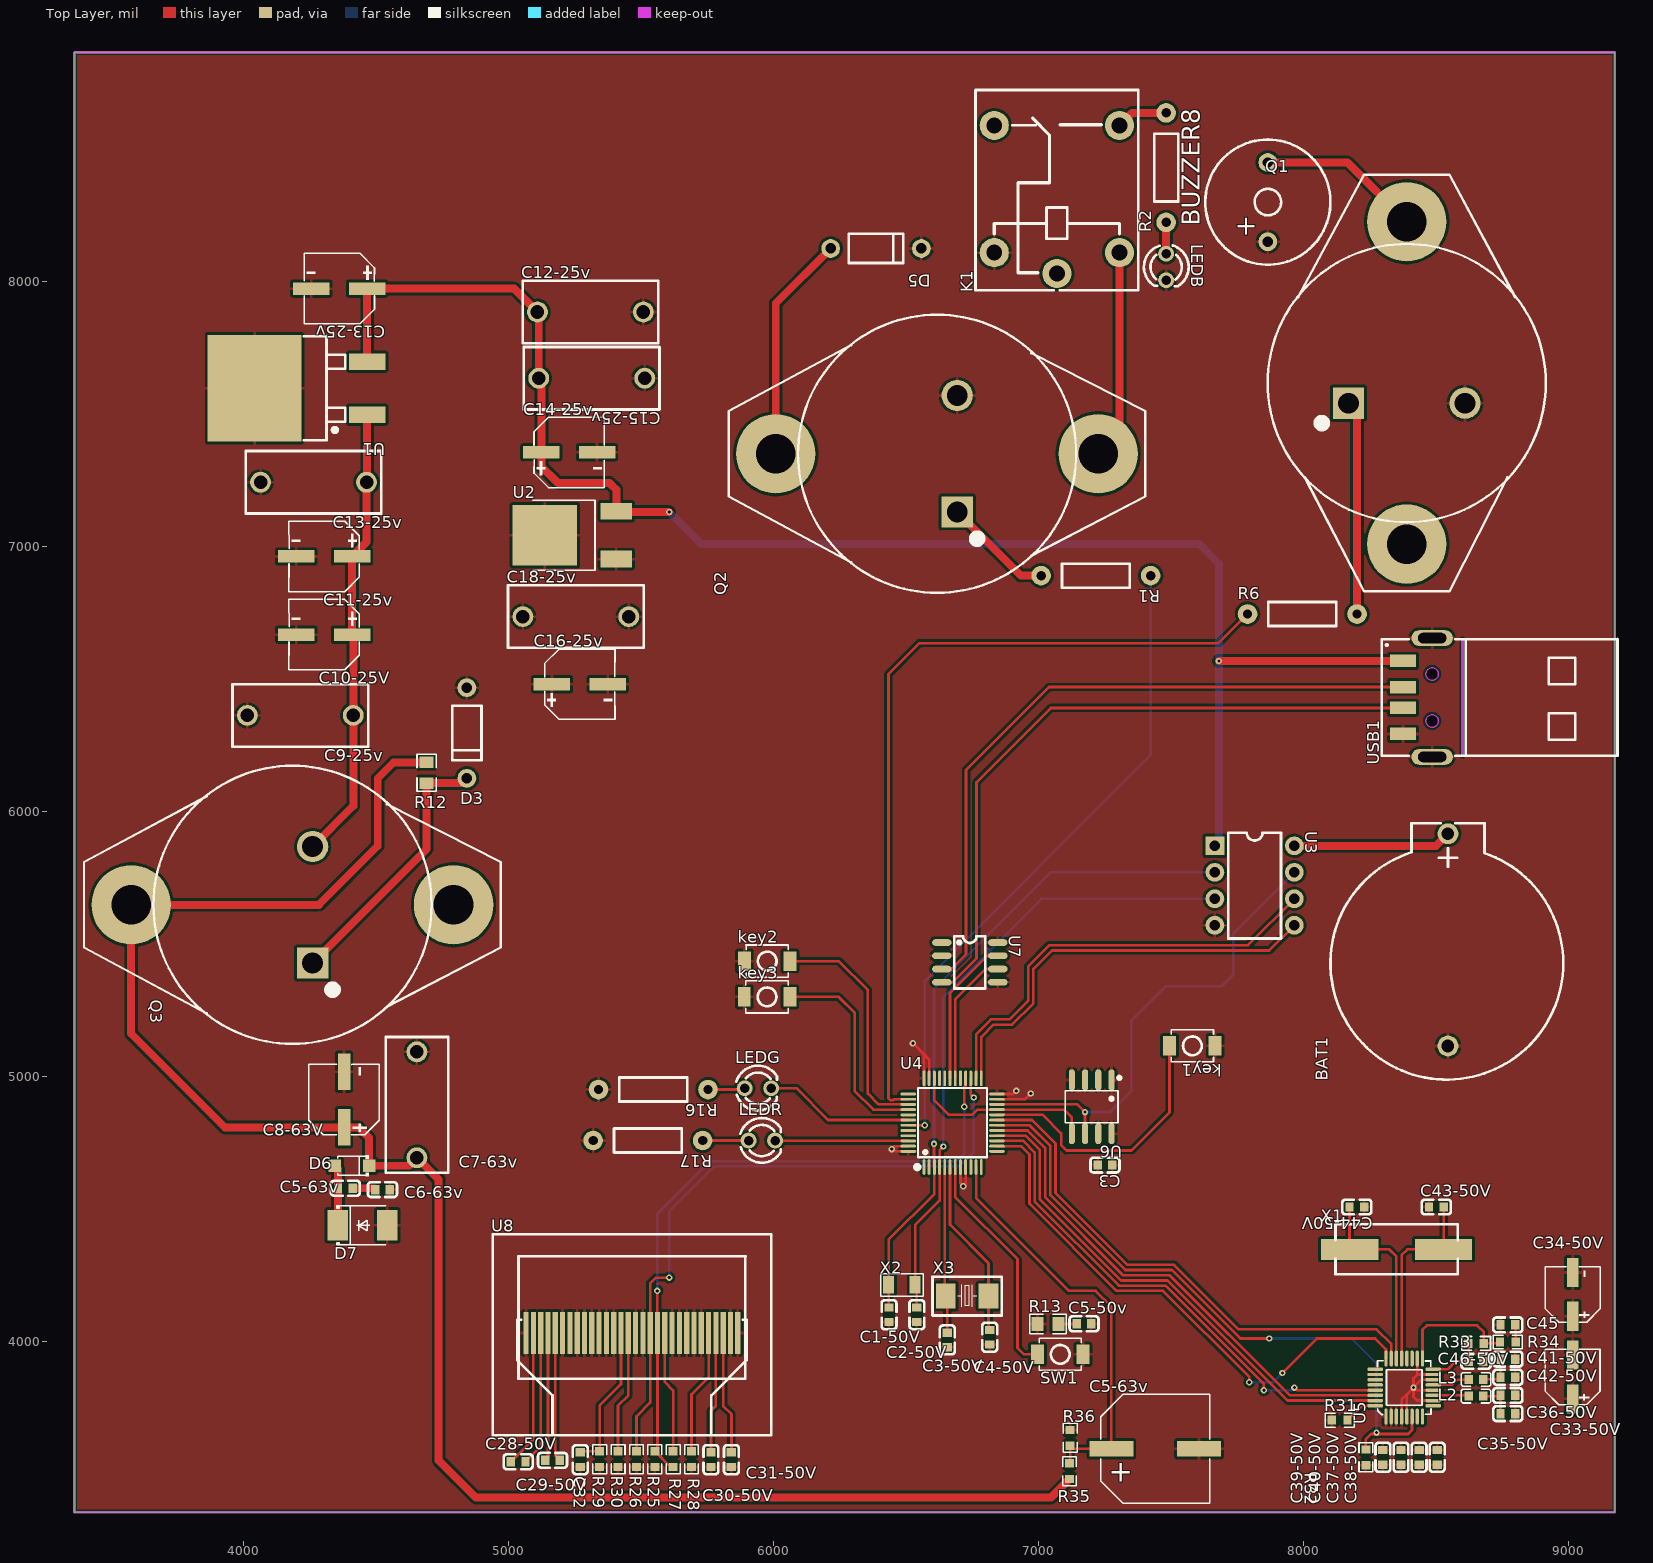
[diagram p0: Top Layer view]
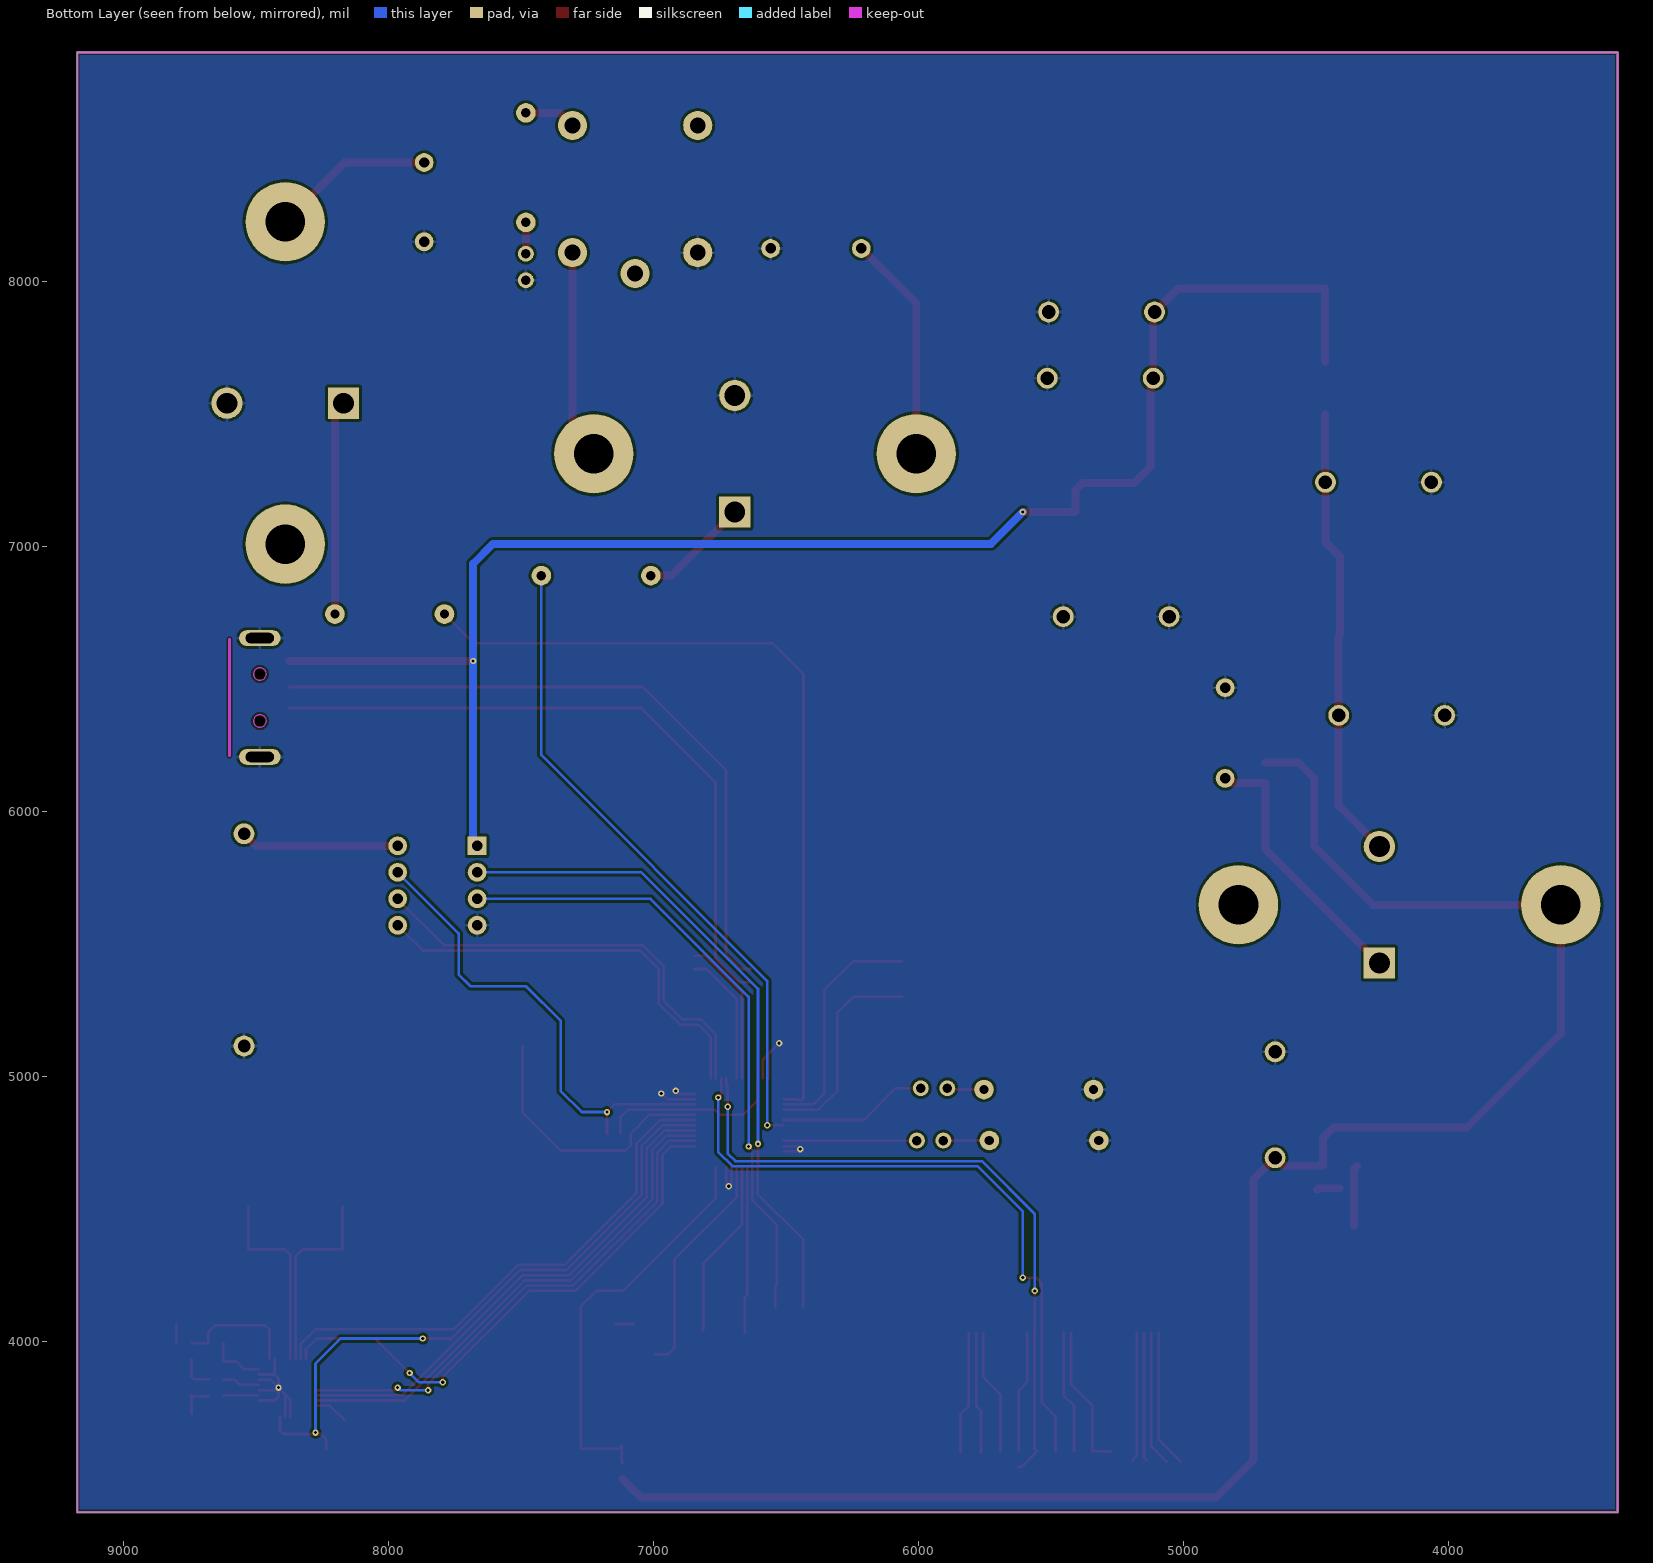
[diagram p1: Bottom Layer view, seen from below]
# Altium PCB MISC52145.pcbdoc
Units mil, origin at the board's own origin, x right, y up, seen from the top; angles counter-clockwise.
Board outline 5815 x 5510 mil, 2 copper layers (Top Layer, Bottom Layer), stack 62.206 mil thick; 90 components, 71 nets, 317 pads, 22 vias.

## Layer stack, top to bottom
Top Solder Mask Layer: solder mask 0.394, Dk 3.3
Top Layer: signal copper 1.379
Dielectric1: surface 59.449, FR4, Dk 4.5
Bottom Layer: signal copper 1.378
Bottom Solder Mask Layer: solder mask 0.394, Dk 3.3

## Board outline
3360,8865 3360,3355 9175,3355 9175,8865

## Design rules (kind name [scope] priority, off if disabled: settings)
BoardOutlineClearance copperThickness2oz_1 [All] p2 off: genericclearance=7.99 ignorepadtopadclearanceinfootprint=FALSE except(0: Arc-SplitContinuation Track-SplitContinuation SMDPad-SplitContinuation THPad-SplitContinuation Via-SplitContinuation Fill-SplitContinuation Region-SplitContinuation Poly-SplitContinuation Text-SplitContinuation Hole-SplitContinuation; 5.98: Arc-CutoutEdge SMDPad-CutoutEdge THPad-CutoutEdge Via-CutoutEdge Fill-CutoutEdge Region-CutoutEdge Text-CutoutEdge; 6.93: Hole-OutlineEdge Hole-CutoutEdge; 10: Poly-OutlineEdge Poly-CutoutEdge; 11.81: Arc-OutlineEdge Track-OutlineEdge SMDPad-OutlineEdge THPad-OutlineEdge Via-OutlineEdge Fill-OutlineEdge Region-OutlineEdge Text-OutlineEdge Track-CutoutEdge)
BoardOutlineClearance Plane_innerPlane_1 [All] p4 off: genericclearance=4.02 ignorepadtopadclearanceinfootprint=FALSE except(0: Arc-SplitContinuation Track-SplitContinuation SMDPad-SplitContinuation THPad-SplitContinuation Via-SplitContinuation Fill-SplitContinuation Region-SplitContinuation Poly-SplitContinuation Text-SplitContinuation Hole-SplitContinuation; 6: SMDPad-CutoutEdge THPad-CutoutEdge Via-CutoutEdge Fill-CutoutEdge Region-CutoutEdge Text-CutoutEdge; 6.93: Hole-OutlineEdge Hole-CutoutEdge; 10: Poly-OutlineEdge Poly-CutoutEdge; 11.8: Arc-OutlineEdge Track-OutlineEdge SMDPad-OutlineEdge THPad-OutlineEdge Via-OutlineEdge Fill-OutlineEdge Region-OutlineEdge Text-OutlineEdge; 11.81: Arc-CutoutEdge Track-CutoutEdge)
BoardOutlineClearance Copper_copperRegion_1 [All] p6 off: genericclearance=4.02 ignorepadtopadclearanceinfootprint=FALSE except(0: Arc-SplitContinuation Track-SplitContinuation SMDPad-SplitContinuation THPad-SplitContinuation Via-SplitContinuation Fill-SplitContinuation Region-SplitContinuation Poly-SplitContinuation Text-SplitContinuation Hole-SplitContinuation; 6: SMDPad-CutoutEdge THPad-CutoutEdge Via-CutoutEdge Fill-CutoutEdge Region-CutoutEdge Text-CutoutEdge; 6.93: Hole-OutlineEdge Hole-CutoutEdge; 10: Poly-OutlineEdge Poly-CutoutEdge; 11.8: Arc-OutlineEdge Track-OutlineEdge SMDPad-OutlineEdge THPad-OutlineEdge Via-OutlineEdge Fill-OutlineEdge Region-OutlineEdge Text-OutlineEdge; 11.81: Arc-CutoutEdge Track-CutoutEdge)
BoardOutlineClearance copperThickness1oz_1 [All] p8: genericclearance=4.02 ignorepadtopadclearanceinfootprint=FALSE except(0: Arc-SplitContinuation Track-SplitContinuation SMDPad-SplitContinuation THPad-SplitContinuation Via-SplitContinuation Fill-SplitContinuation Region-SplitContinuation Poly-SplitContinuation Text-SplitContinuation Hole-SplitContinuation; 6: SMDPad-CutoutEdge THPad-CutoutEdge Via-CutoutEdge Fill-CutoutEdge Region-CutoutEdge Text-CutoutEdge; 6.93: Hole-OutlineEdge Hole-CutoutEdge; 10: Poly-OutlineEdge Poly-CutoutEdge; 11.8: Arc-OutlineEdge Track-OutlineEdge SMDPad-OutlineEdge THPad-OutlineEdge Via-OutlineEdge Fill-OutlineEdge Region-OutlineEdge Text-OutlineEdge; 11.81: Arc-CutoutEdge Track-CutoutEdge)
Clearance copperThickness2oz [All] p1 off: gap=7.99 ignorepadtopadclearanceinfootprint=FALSE except(5.98: SMDPad-Track SMDPad-SMDPad THPad-Track SMDPad-THPad THPad-THPad Track-Via SMDPad-Via THPad-Via Via-Via Fill-Track Region-Track Fill-SMDPad Region-SMDPad Fill-THPad Region-THPad Fill-Via Region-Via Fill-Fill Fill-Region Region-Region Arc-Track Arc-SMDPad Arc-THPad Arc-Via Fill-Arc Region-Arc Arc-Arc Text-Track SMDPad-Text Text-THPad Text-Via Fill-Text Region-Text Arc-Text Text-Text; 6.93: Hole-Track Hole-SMDPad Hole-THPad Hole-Via Fill-Hole Region-Hole Hole-Arc Hole-Text; 10: Poly-Track Poly-SMDPad Poly-THPad Poly-Via Poly-Fill Poly-Region Poly-Poly Poly-Arc Poly-Text Poly-Hole)
Clearance Plane_innerPlane [All] p3 off: gap=4.02 ignorepadtopadclearanceinfootprint=FALSE except(5.98: SMDPad-Track SMDPad-SMDPad THPad-Track SMDPad-THPad THPad-THPad Track-Via SMDPad-Via THPad-Via Via-Via Fill-Track Region-Track Fill-SMDPad Region-SMDPad Fill-THPad Region-THPad Fill-Via Region-Via Fill-Fill Fill-Region Region-Region; 6: Arc-Track Arc-SMDPad Arc-THPad Arc-Via Fill-Arc Region-Arc Arc-Arc Text-Track SMDPad-Text Text-THPad Text-Via Fill-Text Region-Text Arc-Text Text-Text; 6.93: Hole-Track Hole-SMDPad Hole-THPad Hole-Via Fill-Hole Region-Hole Hole-Arc Hole-Text; 10: Poly-Track Poly-SMDPad Poly-THPad Poly-Via Poly-Fill Poly-Region Poly-Poly Poly-Arc Poly-Text Poly-Hole)
Clearance Copper_copperRegion [All] p5 off: gap=4.02 ignorepadtopadclearanceinfootprint=FALSE except(5.98: SMDPad-Track SMDPad-SMDPad THPad-Track SMDPad-THPad THPad-THPad Track-Via SMDPad-Via THPad-Via Via-Via Fill-Track Region-Track Fill-SMDPad Region-SMDPad Fill-THPad Region-THPad Fill-Via Region-Via Fill-Fill Fill-Region Region-Region; 6: Arc-Track Arc-SMDPad Arc-THPad Arc-Via Fill-Arc Region-Arc Arc-Arc Text-Track SMDPad-Text Text-THPad Text-Via Fill-Text Region-Text Arc-Text Text-Text; 6.93: Hole-Track Hole-SMDPad Hole-THPad Hole-Via Fill-Hole Region-Hole Hole-Arc Hole-Text; 10: Poly-Track Poly-SMDPad Poly-THPad Poly-Via Poly-Fill Poly-Region Poly-Poly Poly-Arc Poly-Text Poly-Hole)
Clearance copperThickness1oz [All] p7: gap=4.02 ignorepadtopadclearanceinfootprint=FALSE except(5.98: SMDPad-Track SMDPad-SMDPad THPad-Track SMDPad-THPad THPad-THPad Track-Via SMDPad-Via THPad-Via Via-Via Fill-Track Region-Track Fill-SMDPad Region-SMDPad Fill-THPad Region-THPad Fill-Via Region-Via Fill-Fill Fill-Region Region-Region; 6: Arc-Track Arc-SMDPad Arc-THPad Arc-Via Fill-Arc Region-Arc Arc-Arc Text-Track SMDPad-Text Text-THPad Text-Via Fill-Text Region-Text Arc-Text Text-Text; 6.93: Hole-Track Hole-SMDPad Hole-THPad Hole-Via Fill-Hole Region-Hole Hole-Arc Hole-Text; 10: Poly-Track Poly-SMDPad Poly-THPad Poly-Via Poly-Fill Poly-Region Poly-Poly Poly-Arc Poly-Text Poly-Hole)
DiffPairsRouting differentialPair [All] p1: maxlimit=6 minlimit=6 mostfreqgap=6 toplayer_minwidth=5 toplayer_prefwidth=10 toplayer_maxwidth=100 toplayer_mingap=6 toplayer_prefgap=6 toplayer_maxgap=6 bottomlayer_minwidth=5 bottomlayer_prefwidth=10 bottomlayer_maxwidth=100 bottomlayer_mingap=6 bottomlayer_prefgap=6 bottomlayer_maxgap=6 maxuncoupledlength=10
HoleToHoleClearance otherClearance [All] p1: gap=11.81 allowstackedmicrovias=TRUE
Length netLength [All] p1: minlimit=0 maxlimit=0
PasteMaskExpansion pasteMaskExpansion [All] p1: expansion=0
PlaneConnect innerPlane [All] p1: planeconnectstyle=Relief reliefexpansion=20 reliefentries=4 reliefconductorwidth=10 reliefairgap=10
PolygonConnect copperRegion [(InNet('GND'))] p1: connectstyle=Relief reliefconductorwidth=10 reliefentries=4 polygonreliefangle="90 Angle" airgapwidth=10 via.connectstyle=Relief via.reliefconductorwidth=10 via.reliefentries=4 via.polygonreliefangle="90 Angle" via.airgapwidth=10
RoutingVias viaSize [All] p1: holewidth=12.01 width=24.02 viastyle="Through Hole" minholewidth=11.81 minwidth=19.68 maxholewidth=248.03 maxwidth=393.7
SolderMaskExpansion solderMaskExpansion [IsVia] p1: expansion=-1000 istentingtop=TRUE
SolderMaskExpansion solderMaskExpansion [All] p2: expansion=2 istentingtop=FALSE
Width copperThickness2oz_2 [All] p1 off: maxlimit=100 minlimit=8 preferedwidth=10
Width copperThickness1oz_2 [All] p2: maxlimit=100 minlimit=5 preferedwidth=10

## Components (designator, comment, footprint, x,y, rotation, side; value= is the part's Value field where it differs from the comment)
BAT1 "CR2032-2-1" BAT-TH_CR2032-2-1 8545,5515 r90 top
BUZZER8 "buzzer-12X9" BUZ-TH_BD12.0-P7.60-D0.6-FD 7865,8300 r90 top
C1-50V "22pF" C0603 6435,4100 r270 top
C2-50V "22pF" C0603 6540,4100 r270 top
C3 "100nF" C0603 7250,4665 r180 top
C3-50V "22pF" C0603 6655,4005 r270 top
C4-50V "22pF" C0603 6815,4015 r270 top
C5-50v "100nF" C0603 7171.16,4065.82 r0 top
C5-63v "100uF" CAP-SMD_BD10.0-L10.3-W10.3-LS11.0-FD_1 7439.75,3593.72 r0 top
C5-63v "100nF" C0603 4382.66,4577.44 r180 top
C6-63v "100nF" C0603 4522.66,4572.44 r180 top
C7-63v "100nF" CAP-TH_L13.0-W6.0-P10.00-D1.0 4652.66,4892.44 r90 top
C8-63V "100uF" CAP-SMD_BD6.3-L6.6-W6.6-LS7.3-FD-H7.7 4377.66,4912.44 r90 top
C9-25v "100nF" CAP-TH_L13.0-W6.0-P10.00-D1.0 4212.66,6362.44 r180 top
C10-25V "100uF" CAP-SMD_BD6.3-L6.6-W6.6-LS7.3-FD-H7.7 4302.66,6667.44 r180 top
C11-25v "100uF" CAP-SMD_BD6.3-L6.6-W6.6-LS7.3-FD-H7.7 4302.66,6962.44 r180 top
C12-25v "100nF" CAP-TH_L13.0-W6.0-P10.00-D1.0 5307.66,7885.24 r0 top
C13-25v "100uF" CAP-SMD_BD6.3-L6.6-W6.6-LS7.3-FD-H7.7 4359.68,7973.62 r180 top
C13-25v "100nF" CAP-TH_L13.0-W6.0-P10.00-D1.0 4262.66,7242.44 r180 top
C14-25v "100uF" CAP-SMD_BD6.3-L6.6-W6.6-LS7.3-FD-H7.7 5227.66,7355.24 r0 top
C15-25v "100nF" CAP-TH_L13.0-W6.0-P10.00-D1.0 5312.66,7635.24 r180 top
C16-25v "100uF" CAP-SMD_BD6.3-L6.6-W6.6-LS7.3-FD-H7.7 5267.66,6480.24 r0 top
C18-25v "100nF" CAP-TH_L13.0-W6.0-P10.00-D1.0 5252.66,6735.24 r0 top
C28-50V "1uF" C0603 5035,3545 r180 top
C29-50V "1uF" C0603 5164.81,3550.37 r180 top
C30-50V "4.7uF" C0603 5762.84,3552.81 r90 top
C31-50V "2.2uF" C0603 5840.08,3552.81 r90 top
C32 "10uF" C0603 5269.49,3552.81 r90 top
C33-50V "0.1uF" CAP-SMD_BD5.0-L5.3-W5.3-FD 9015.85,3865.07 r90 top
C34-50V "0.1uF" CAP-SMD_BD5.0-L5.3-W5.3-FD 9015.91,4176.73 r90 top
C35-50V "47pF" C0603 8770.92,3795.31 r180 top
C36-50V "15pF" C0603 8770.91,3726.73 r0 top
C37-50V "180pF" C0603 8435.96,3561.73 r90 top
C38-50V "10pF" C0603 8504.27,3561.73 r90 top
C39-50V "180pF" C0603 8299.36,3561.73 r90 top
C40-50V "10pF" C0603 8367.66,3561.73 r90 top
C41-50V "15pF" C0603 8770.91,3932.47 r0 top
C42-50V "47pF" C0603 8770.91,3863.89 r0 top
C43-50V "15pF" C0603 8500.91,4506.73 r0 top
C44-50V "15pF" C0603 8200.91,4506.73 r180 top
C45 "0.1uF" C0603 8770.91,4061.73 r0 top
C46-50V "0.1uF" C0603 8650.91,3923.61 r0 top
D3 "1N4742A" DO-41_BD2.4-L4.7-P8.70-D0.9-RD 4841.4,6295.87 r90 top
D5 "1N4003-E3/54" DO-41_BD2.4-L4.7-P8.70-D0.9-RD 6385.95,8125.05 r180 top
D6 "1N4003W" SOD-123FL_L2.7-W1.8-LS3.8-RD 4407.66,4662.44 r180 top
D7 "SMBJ51A" SMB_L4.3-W3.6-LS5.4-R-RD 4447.66,4437.44 r0 top
K1 "" RELAY-TH_SRD-DCXXV-SL-C 7068.54,8310.03 r90 top
key1 "TS-1088-AR02016" SW-SMD_L3.9-W3.0-P4.45 7580,5115 r180 top
key2 "TS-1088-AR02016" SW-SMD_L3.9-W3.0-P4.45 5975,5435 r0 top
key3 "TS-1088-AR02016" SW-SMD_L3.9-W3.0-P4.45 5974.59,5299.8 r0 top
L2 "2.2uH" L0603 8650.91,3792.51 r0 top
L3 "2.2uH" L0603 8650.91,3855.91 r0 top
LEDB "" LED_TH-3mm 7480.95,8055.05 r270 top
LEDG "" LED_TH-3mm 5940,4955 r0 top
LEDR "" LED_TH-3mm 5954.79,4757.59 r0 top
Q1 "2N3055" TO-3_L39.4-W26.7-P10.92-BL 8389.2,7617.41 r0 top
Q2 "2N3055" TO-3_L39.4-W26.7-P10.92-BL 6615.95,7350.05 r90 top
Q3 "2N3055" TO-3_L39.4-W26.7-P10.92-BL 4182.66,5647.44 r90 top
R1 "" RES-TH_BD2.3-L6.5-P10.50-D0.5 7215.95,6890.05 r180 top
R2 "" RES-TH_BD2.3-L6.5-P10.50-D0.5 7480.95,8430.05 r90 top
R6 "" RES-TH_BD2.3-L6.5-P10.50-D0.5 7995,6745 r0 top
R12 "10kΩ" R0805 4689.17,6145.87 r90 top
R13 "10kΩ" R0805 7035,4065 r0 top
R16 "" RES-TH_BD2.3-L6.5-P10.50-D0.5 5545,4950 r180 top
R17 "" RES-TH_BD2.3-L6.5-P10.50-D0.5 5524.79,4757.63 r180 top
R25 "4.7K" R0603 5550.84,3555 r270 top
R26 "4.7K" R0603 5481.49,3555 r270 top
R27 "0" R0603 5620.19,3555 r90 top
R28 "910K" R0603 5689.54,3555 r90 top
R29 "10K" R0603 5342.79,3555 r270 top
R30 "10K" R0603 5412.14,3555 r270 top
R31 "1K" R0603 8135.91,3701.73 r0 top
R32 "10k" R0603 8235,3561.73 r270 top
R33 "820Ω" R0603 8650.91,3991.73 r0 top
R34 "5.1k" R0603 8770.92,3997.1 r0 top
R35 "30kΩ" R0603 7116.37,3509.66 r90 top
R36 "1kΩ" R0603 7118.81,3635.34 r270 top
SW1 "TS-1088-AR02016" SW-SMD_L3.9-W3.0-P4.45 7081.16,3950.56 r0 top
U1 "L7805ABD2T-TR" TO-263-2_L10.0-W9.2-P5.08-LS15.3-TL-CW 4252.66,7597.44 r180 top
U2 "LD1117DT33TR" TO-252-2_L6.6-W6.1-P4.57-LS9.9-BR-CW 5270.71,7042.64 r0 top
U3 "DS1302" DIP-8_L9.7-W6.4-P2.54-LS7.6-BL 7815,5720 r270 top
U4 "STM32F103C8T6" LQFP-48_L7.0-W7.0-P0.50-LS9.0-BL 6675,4825 r0 top
U5 "MFRC522" QFN32 8310.91,3716.73 r90 top
U6 "AT24C02" SOIC-8_L4.9-W3.9-P1.27-LS6.0-BL 7200,4885 r180 top
U7 "CH340N" SOP-8_L4.9-W3.9-P1.27-LS6.0-BL 6740,5430 r270 top
U8 "X096-2864KLBAG01-H30" OLED-SMD_X096-2864KLBAG01-H30 5464.46,4030.95 r0 top
USB1 "U217-041N-4BV81" USB-A-SMD_U217-041N-4BV81 8430,6430 r90 top
X1 "27.12MHz" OSC-SMD_L11.4-W4.5-LS12.5 8350.91,4346.73 r0 top
X2 "32.768kHz" CRYSTAL-SMD_L3.2-W1.5-1 6483.58,4212.95 r180 top
X3 "8MHz" CRYSTAL-SMD_L5.0-W3.2 6730,4170 r180 top

## Footprints (in the part's own frame and the unit in brackets; to place one, negate y for a bottom-side part, rotate by r counter-clockwise, add the part's x,y. Pads: shape width x height; smd on the part's side, far side on the other; paste and mask are expansions set on the pad)
BAT-TH_CR2032-2-1 [mm]
  round 2 hole 1.2 paste+0 mask+0.051: 1(10.175,0) 2(-10.175,0)
  silkscreen extent -13.4,-11.05 11.17,11.26
BUZ-TH_BD12.0-P7.60-D0.6-FD [mil]
  round 70.9 hole 39.4 paste+0 mask+2: 1(-149.6,0) 2(149.6,0)
  silkscreen extent -236,-236 236,236
C0603 [mm]
  rect 0.8x0.9 smd: 1(-0.7,0) 2(0.7,0)
  silkscreen extent -1.39,-0.71 1.39,0.71
CAP-SMD_BD5.0-L5.3-W5.3-FD [mm]
  rect 2.8x1.1 smd: 1(-2.1,0) 2(2.1,0)
  silkscreen extent -2.66,-2.62 2.66,2.65
CAP-SMD_BD6.3-L6.6-W6.6-LS7.3-FD-H7.7 [mm]
  rect 3.5x1.2 smd: 1(-2.67,0) 2(2.67,0)
  silkscreen extent -3.38,-3.38 3.38,3.38
CAP-SMD_BD10.0-L10.3-W10.3-LS11.0-FD_1 [mm]
  rect 4.2x1.5 smd: 1(-4.2,0) 2(4.2,0)
  silkscreen extent -5.23,-5.23 5.23,5.23
CAP-TH_L13.0-W6.0-P10.00-D1.0 [mm]
  round 2 hole 1.3: 1(-5.08,0) 2(5.08,0)
  silkscreen extent -6.5,-3 6.5,3
CRYSTAL-SMD_L3.2-W1.5-1 [mm]
  rect 1.05x1.7 smd: 1(-1.275,0) 2(1.275,0)
  silkscreen extent -2.03,-1.08 2.03,1.08
CRYSTAL-SMD_L5.0-W3.2 [mm]
  rect 1.9x2.4 smd: 1(-2.05,0) 2(2.05,0)
  silkscreen extent -3.32,-1.85 3.33,1.85
DIP-8_L9.7-W6.4-P2.54-LS7.6-BL [mm]
  rect 1.8x1.8 hole 1 paste+0 mask+0.05: 1(-3.81,-3.81)
  round 1.8 hole 1 paste+0 mask+0.05: 2(-1.27,-3.81) 3(1.27,-3.81) 4(3.81,-3.81) 5(3.81,3.81) 6(1.27,3.81) 7(-1.27,3.81) 8(-3.81,3.81)
  silkscreen extent -5.08,-2.53 5.08,2.53
DO-41_BD2.4-L4.7-P8.70-D0.9-RD [mm]
  round 1.8 hole 1: 1(-4.35,0) 2(4.35,0)
  silkscreen extent -2.6,-1.4 2.6,1.4
L0603 [mm]
  rect 0.8x0.864 smd paste-100 mask+0.051: 1(-0.7,0) 2(0.7,0)
  silkscreen extent -1.42,-0.65 1.42,0.65
LED_TH-3mm [mil]
  round 60 hole 36 paste+0 mask+2: 1(-50,0) 2(50,0)
  silkscreen extent -81,-84 72,85
LQFP-48_L7.0-W7.0-P0.50-LS9.0-BL [mm]
  oval 0.27x1.5 smd paste+0 mask+0.05: 1(-2.75,-4.25) 2(-2.25,-4.25) 3(-1.75,-4.25) 4(-1.25,-4.25) 5(-0.75,-4.25) 6(-0.25,-4.25) 7(0.25,-4.25) 8(0.75,-4.25) 9(1.25,-4.25) 10(1.75,-4.25) 11(2.25,-4.25) 12(2.75,-4.25) 25(2.75,4.25) 26(2.25,4.25) 27(1.75,4.25) 28(1.25,4.25) 29(0.75,4.25) 30(0.25,4.25) 31(-0.25,4.25) 32(-0.75,4.25) 33(-1.25,4.25) 34(-1.75,4.25) 35(-2.25,4.25) 36(-2.75,4.25)
  oval 1.5x0.27 smd paste+0 mask+0.05: 13(4.25,-2.75) 14(4.25,-2.25) 15(4.25,-1.75) 16(4.25,-1.25) 17(4.25,-0.75) 18(4.25,-0.25) 19(4.25,0.25) 20(4.25,0.75) 21(4.25,1.25) 22(4.25,1.75) 23(4.25,2.25) 24(4.25,2.75) 37(-4.25,2.75) 38(-4.25,2.25) 39(-4.25,1.75) 40(-4.25,1.25) 41(-4.25,0.75) 42(-4.25,0.25) 43(-4.25,-0.25) 44(-4.25,-0.75) 45(-4.25,-1.25) 46(-4.25,-1.75) 47(-4.25,-2.25) 48(-4.25,-2.75)
  silkscreen extent -3.59,-4.46 3.3,3.34
OLED-SMD_X096-2864KLBAG01-H30 [mm]
  rect 0.5x4 smd: 1(-10.15,0) 2(-9.45,0) 3(-8.75,0) 4(-8.05,0) 5(-7.35,0) 6(-6.65,0) 7(-5.95,0) 8(-5.25,0) 9(-4.55,0) 10(-3.85,0) 11(-3.15,0) 12(-2.45,0) 13(-1.75,0) 14(-1.05,0) 15(-0.35,0) 16(0.35,0) 17(1.05,0) 18(1.75,0) 19(2.45,0) 20(3.15,0) 21(3.85,0) 22(4.55,0) 23(5.25,0) 24(5.95,0) 25(6.65,0) 26(7.35,0) 27(8.05,0) 28(8.75,0) 29(9.45,0) 30(10.15,0)
  silkscreen extent -13.35,-9.8 13.35,9.46
OSC-SMD_L11.4-W4.5-LS12.5 [mm]
  rect 5.5x2 smd: 1(-4.5,0) 2(4.5,0)
  silkscreen extent -5.85,-2.4 5.85,2.4
QFN32 [mil]
  oval 60x13 smd: 1(-1,0) 2(-1,-20) 3(-1,-39.39) 4(-1,-59.08) 5(-1,-78.76) 6(-1,-98.45) 7(-1,-118.15) 8(-1,-137.84) 17(218,-137.84) 18(218,-118.15) 19(218,-98.45) 20(218,-78.76) 21(218,-59.08) 22(218,-39.39) 23(218,-20) 24(218,0)
  oval 13x60 smd: 9(39.59,-178.42) 10(59.28,-178.42) 11(78.97,-178.42) 12(98.66,-178.42) 13(118.35,-178.42) 14(138.04,-178.42) 15(157.73,-178.42) 16(177.38,-178.42) 25(177.38,40.58) 26(157.73,40.58) 27(138.04,40.58) 28(118.35,40.58) 29(98.66,40.58) 30(78.97,40.58) 31(59.28,40.58) 32(39.59,40.58)
  silkscreen extent 6,-169 210,32
R0603 [mil]
  rect 31.75x34.02 smd paste-3937.01 mask+2: 1(-29.66,0) 2(29.66,0)
  silkscreen extent -55,-26 55,26
R0805 [mm]
  rect 1.133x1.377 smd paste-100 mask+0.051: 1(-1,0) 2(1,0)
  silkscreen extent -1.76,-0.92 1.76,0.92
RELAY-TH_SRD-DCXXV-SL-C [mil]
  round 110 hole 60 paste+0 mask+2: 1(-200.8,-236.2) 2(279.5,-236.2) 3(279.5,236.2) 4(-200.8,236.2) 5(-279.5,0)
  silkscreen extent -343,-307 413,307
RES-TH_BD2.3-L6.5-P10.50-D0.5 [mil]
  round 74 hole 35.4 paste+0 mask+2: 1(-206.69,0) 2(206.69,0)
  silkscreen extent -128,-45 128,45
SMB_L4.3-W3.6-LS5.4-R-RD [mm]
  rect 1.96x2.94 smd: 1(2.38,0) 2(-2.38,0)
  silkscreen extent -2.49,-1.88 2.23,1.88
SOD-123FL_L2.7-W1.8-LS3.8-RD [mm]
  rect 1.2x1.2 smd: 1(-1.635,0) 2(1.635,0)
  silkscreen extent -1.6,-1 1.38,1
SOIC-8_L4.9-W3.9-P1.27-LS6.0-BL [mm]
  oval 0.588x2.045 smd: 1(-1.905,-2.57) 2(-0.635,-2.57) 3(0.635,-2.57) 4(1.905,-2.57) 5(1.905,2.57) 6(0.635,2.57) 7(-0.635,2.57) 8(-1.905,2.57)
  silkscreen extent -2.8,-2.92 2.53,1.52
SOP-8_L4.9-W3.9-P1.27-LS6.0-BL [mm]
  oval 0.63x1.865 smd: 1(-1.905,-2.682) 2(-0.635,-2.682) 3(0.635,-2.682) 4(1.905,-2.682) 5(1.905,2.682) 6(0.635,2.682) 7(-0.635,2.682) 8(-1.905,2.682)
  silkscreen extent -2.5,-1.5 2.5,1.48
SW-SMD_L3.9-W3.0-P4.45 [mm]
  rect 1.23x1.86 smd: 1(-2.185,0) 2(2.185,0)
  silkscreen extent -2.03,-1.54 2.03,1.54
TO-3_L39.4-W26.7-P10.92-BL [mil]
  rect 118.11x118.11 hole 78.74: 1(-220,-76.5)
  round 118.11 hole 78.74: 2(220,-76.5)
  round 300 hole 150: 3(0,608.5) 4(0,-608.5)
  silkscreen extent -525,-786 525,786
TO-252-2_L6.6-W6.1-P4.57-LS9.9-BR-CW [mm]
  rect 3x1.6 smd: 1(3.424,-2.29) 3(3.424,2.29)
  rect 6.2x5.8 smd: 2(-3.424,0)
  silkscreen extent -4.58,-3.35 1.38,3.35
TO-263-2_L10.0-W9.2-P5.08-LS15.3-TL-CW [mm]
  rect 3.5x1.6 smd: 1(-5.397,2.54) 3(-5.397,-2.54)
  rect 9x10.2 smd: 2(5.397,0)
  silkscreen extent -3.3,-5 0.67,5
USB-A-SMD_U217-041N-4BV81 [mil]
  rect 47.2x98.4 smd paste-3937.01 mask+2: 1(137.8,55.1) 2(39.4,55.1) 3(-39.4,55.1) 4(-137.8,55.1)
  oval 59.1x157.5 hole 39.4 slot 106.3 at 90 deg paste+0 mask+2: 5(-224.4,-55.1) 6(224.4,-55.1)
  Board Outline Layer circle w0.1: c-88.6,-55.1 r23.6
  Board Outline Layer circle w0.1: c88.6,-55.1 r23.6
  Board Outline Layer lines w10: -220,-170 220,-170
  Board Outline Layer region: -88.6,-78.7 -98.84,-76.36 -107.05,-69.81 -111.61,-60.35 -111.61,-49.85 -107.05,-40.39 -98.84,-33.84 -88.6,-31.5 -88.6,-31.5 -78.36,-33.84 -70.15,-40.39 -65.59,-49.85 -65.59,-60.35 -70.15,-69.81 -78.36,-76.36 -88.6,-78.7
  Board Outline Layer region: -88.6,-78.7 -92.7,-78.34 -96.67,-77.28 -100.4,-75.54 -103.77,-73.18 -106.68,-70.27 -109.04,-66.9 -110.78,-63.17 -111.84,-59.2 -112.2,-55.1 -111.84,-51 -110.78,-47.03 -109.04,-43.3 -106.68,-39.93 -103.77,-37.02 -100.4,-34.66 -96.67,-32.92 -92.7,-31.86 -88.6,-31.5 -84.5,-31.86 -80.53,-32.92 -76.8,-34.66 -73.43,-37.02 -70.52,-39.93 -68.16,-43.3 -66.42,-47.03 -65.36,-51 -65,-55.1 -65.36,-59.2 -66.42,-63.17 -68.16,-66.9 -70.52,-70.27 -73.43,-73.18 -76.8,-75.54 -80.53,-77.28 -84.5,-78.34
  Board Outline Layer region: 88.6,-78.7 78.36,-76.36 70.15,-69.81 65.59,-60.35 65.59,-49.85 70.15,-40.39 78.36,-33.84 88.6,-31.5 88.6,-31.5 98.84,-33.84 107.05,-40.39 111.61,-49.85 111.61,-60.35 107.05,-69.81 98.84,-76.36 88.6,-78.7
  Board Outline Layer region: 88.6,-78.7 84.5,-78.34 80.53,-77.28 76.8,-75.54 73.43,-73.18 70.52,-70.27 68.16,-66.9 66.42,-63.17 65.36,-59.2 65,-55.1 65.36,-51 66.42,-47.03 68.16,-43.3 70.52,-39.93 73.43,-37.02 76.8,-34.66 80.53,-32.92 84.5,-31.86 88.6,-31.5 92.7,-31.86 96.67,-32.92 100.4,-34.66 103.77,-37.02 106.68,-39.93 109.04,-43.3 110.78,-47.03 111.84,-51 112.2,-55.1 111.84,-59.2 110.78,-63.17 109.04,-66.9 106.68,-70.27 103.77,-73.18 100.4,-75.54 96.67,-77.28 92.7,-78.34
  Multi-Layer board cut-out: -88.6,-78.7 -98.84,-76.36 -107.05,-69.81 -111.61,-60.35 -111.61,-49.85 -107.05,-40.39 -98.84,-33.84 -88.6,-31.5 -88.6,-31.5 -78.36,-33.84 -70.15,-40.39 -65.59,-49.85 -65.59,-60.35 -70.15,-69.81 -78.36,-76.36 -88.6,-78.7
  Multi-Layer board cut-out: 88.6,-78.7 78.36,-76.36 70.15,-69.81 65.59,-60.35 65.59,-49.85 70.15,-40.39 78.36,-33.84 88.6,-31.5 88.6,-31.5 98.84,-33.84 107.05,-40.39 111.61,-49.85 111.61,-60.35 107.05,-69.81 98.84,-76.36 88.6,-78.7
  silkscreen extent -220,-755 221,135

## Via types
v1: diameter 24.02, hole 12, Top Layer to Bottom Layer, 22 vias

## Nets (pads, with @x,y where several pads share a name; then routed paths per layer and width w, separated by ;. In a path a pad name is that pad's centre, name@x,y a point inside that pad or via, vN(x,y) a via of type N, cw(c..) or ccw(c..) an arc to the next point about the centre after c; other vN are vias at no path point)
48V: C7-63v.1 C8-63V.1 D6.1 Q3.3 R12.2 R35.1 | length 6977.9
  Top Layer w30: R12.2 4565.24,6185.24 4505,6125 4505,5870 4282.44,5647.44 Q3.3 3574.16,5160.84 3927.68,4807.32 C8-63V.1 4432.68,4807.32 4472.03,4767.97 D6.1 4622.66,4662.44 C7-63v.1 4735,4610.1 4735,3550 4875,3410 7046.37,3410 R35.1
$1N38859: C9-25v.1 C10-25V.1 C11-25v.1 C13-25v.1@4462.66,7242.44 Q3.2 U1.1 | length 1719.4
  Top Layer w30: Q3.2 4412.66,6020.94 C9-25v.1 4412.66,6662.56 C10-25V.1 C11-25v.1 4462.66,7017.32 4462.66,7242.44 4465.16,7244.94 U1.1
$1N38873: LEDR.1 R17.1 | length 173.3
  Top Layer w10: R17.1 LEDR.1
$1N38876: Q1.1 R6.2 | length 809.4
  Top Layer w30: Q1.1 8201.69,7508.42 R6.2
$1N38881: U7.4 USB1.3 | length 2559
  Top Layer w10: U7.4 6675,5355 6765,5445 6765,6110 7045.6,6390.6 USB1.3
$1N38882: U7.3 USB1.2 | length 2588.5
  Top Layer w10: U7.3 6670,5405 6725.6,5460.6 6725.6,6155.6 7039.4,6469.4 USB1.2
$1N38894: C5-50v.1 R13.2 | length 69.6
  Top Layer w10: R13.2 7142.78,4065 C5-50v.1
$1N38907: C35-50V.2 C36-50V.1 L2.2 | length 134.6
  Top Layer w10: L2.2 8740.56,3792.51 C35-50V.2 C36-50V.1
$1N38908: L2.1 U5.11 | length 135.3
  Top Layer w10: U5.11 8620.18,3795.69 L2.1
$1N38909: C41-50V.1 C42-50V.1 L3.2 | length 136.8
  Top Layer w10: L3.2 8735.37,3855.91 C42-50V.1 C41-50V.1
$1N38910: L3.1 U5.13 | length 142.7
  Top Layer w10: U5.13 8560.07,3835.07 8580,3855 8622.45,3855 L3.1
$1N38911: C43-50V.2 U5.21 X1.2 | length 717.5
  Top Layer w10: U5.21 8369.99,4324.99 8391.73,4346.73 X1.2 8528.47,4347.12 C43-50V.2
$1N38912: C44-50V.2 U5.22 X1.1 | length 732.9
  Top Layer w10: C44-50V.2 8173.35,4347.12 X1.1 8323.27,4346.73 8350.3,4319.7 U5.22
$1N38913: C45.2 R34.2 | length 65.5
  Top Layer w10: C45.2 8800.58,4059.63 R34.2
$1N38914: C46-50V.1 R33.1 U5.16 | length 215.2
  Top Layer w10: U5.16 8544.11,3894.11 8573.61,3923.61 C46-50V.1 8623.35,3989.63 R33.1
$1N38915: R31.2 U5.32 | length 127.4
  Top Layer w10: R31.2 8220.16,3756.31 U5.32
$1N38917: R33.2 R34.1 U5.17 | length 463.6
  Top Layer w10: U5.17 8448.75,4043.75 8465,4060 8655,4060 8680.57,4034.43 R33.2 8736.25,3991.73 R34.1@8741.25,3996.73
$1N38924: C28-50V.2 U8.2 | length 521.1
  Top Layer w10: C28-50V.2 5092.4,3629.96 U8.2
$1N38925: C28-50V.1 U8.3 | length 509.7
  Top Layer w10: C28-50V.1 5119.96,3602.4 U8.3
$1N38926: C29-50V.2 U8.4 | length 484.8
  Top Layer w10: C29-50V.2 5147.52,3560.65 U8.4
$1N38927: C29-50V.1 U8.5 | length 487.7
  Top Layer w10: U8.5 5175.08,3567.65 C29-50V.1
$1N38932: R30.1 U8.15 | length 462.3
  Top Layer w10: R30.1 5412.14,3757.14 5450.67,3795.67 U8.15
$1N38936: R27.2 U8.20 | length 459.4
  Top Layer w10: U8.20 5588.47,3846.53 5620.19,3814.81 R27.2
$1N38938: R28.2 U8.26 | length 472.9
  Top Layer w10: R28.2 5689.54,3799.54 5753.82,3863.82 U8.26
$1N38939: C30-50V.2 U8.27 | length 458.3
  Top Layer w10: C30-50V.2 5762.84,3737.84 5781.38,3756.38 U8.27
$1N38940: C31-50V.2 U8.28 | length 463.5
  Top Layer w10: U8.28 5808.94,3756.06 5840.08,3724.92 C31-50V.2
$1N38951: D5.2 Q2.3 | length 860.8
  Top Layer w30: Q2.3 6007.45,7917.81 D5.2
$1N38952: K1.1 Q2.4 | length 792.4
  Top Layer w30: Q2.4 7304.74,7430.34 K1.1
$1N38954: Q2.1 R1.2 | length 416.2
  Top Layer w30: Q2.1 6932.45,6890.05 R1.2
$1N38957: C5-63v.1@4410.22,4577.44 C6-63v.2 | length 87
  Top Layer w30: C5-63v.1@4410.22,4577.44 4490.1,4577.44 C6-63v.2
$1N38960: LEDG.1 R16.1 | length 140.4
  Top Layer w10: R16.1 5885,4950 LEDG.1
$1N38962: K1.2 R2.2 | length 195.8
  Top Layer w30: K1.2 7351.95,8636.74 R2.2
$1N38964: K1.5
$1N38967: BUZZER8.2 Q1.3 | length 616.9
  Top Layer w30: BUZZER8.2 8165.51,8449.6 Q1.3
$1N39008: D3.1 Q3.1 R12.1 | length 1016.9
  Top Layer w30: Q3.1 4689.17,5857.46 R12.1 4823.29,6106.5 D3.1
$1N39011: LEDB.1 R2.1 | length 118.3
  Top Layer w30: LEDB.1 R2.1
$1N39016: BAT1.1 U3.8 | length 598.9
  Top Layer w30: U3.8 8499.41,5870 BAT1.1
+5V: C12-25v.1 C13-25v.1@4464.8,7973.62 C14-25v.1 C15-25v.2 U1.3 U2.3 U3.1 USB1.1 | length 6068.4
  Top Layer w30: U1.3 4465.16,7973.26 4464.8,7973.62 5019.27,7973.62 C12-25v.1 5112.66,7880.24 C15-25v.2 5122.54,7625.36 C14-25v.1 5122.54,7302.46 5185,7240 5380,7240 5405.51,7214.49 U2.3 5408.31,7130 v1(5605,7130) ; v1(7680,6567.8) USB1.1
  Bottom Layer w30: v1(5605,7130) 5725,7010 7605,7010 7680,6935 v1(7680,6567.8) 7680,5885 U3.1
ADC: C5-63v.1@7274.39,3593.71 R35.2 R36.2 U4.11 | length 1562
  Top Layer w10: U4.11 6763.58,4541.42 7115,4190 7215,4190 7274.39,4130.61 7274.39,3593.71 7130.77,3593.71 R36.2 7118.81,3541.75 R35.2
BUZZ: R6.1 U4.38 | length 3129.5
  Top Layer w10: U4.38 6453.58,4913.58 6450,4910 6440,4910 6432.93,4917.07 6432.93,6517.93 6550,6635 7678.31,6635 R6.1
GND: BAT1.2 BUZZER8.1 C1-50V.2 C2-50V.2 C3-50V.2 C3.1 C3.2 C4-50V.2 C5-50v.2 C5-63v.2@7605.1,3593.71 C6-63v.1 C7-63v.2 C8-63V.2 C9-25v.2 C10-25V.2 C11-25v.2 C12-25v.2 C13-25v.2 C14-25v.2 C15-25v.1 C16-25v.1 C16-25v.2 C18-25v.1 C18-25v.2 C30-50V.1 C31-50V.1 C32.1 C33-50V.1 C33-50V.2 C34-50V.1 C34-50V.2 C35-50V.1 C36-50V.2 C37-50V.1 C37-50V.2 C38-50V.1 C38-50V.2 C39-50V.1 C39-50V.2 C40-50V.1 C40-50V.2 C41-50V.2 C42-50V.2 C43-50V.1 C44-50V.1 C45.1 C46-50V.2 D3.2 D5.1 D7.1 K1.4 key1.1 key2.1 key3.1 LEDB.2 Q1.2 Q2.2 R13.1 R16.2 R17.2 R25.2 R26.2 R28.1 R29.2 R30.2 R31.1 R32.2 R36.1 SW1.2 U1.2 U2.1 U2.2 U3.4 U4.8 U4.9 U4.23 U4.24 U4.35 U4.36 U4.47 U4.48 U5.1 U5.2 U5.3 U5.4 U5.5 U5.10 U5.12 U5.14 U5.15 U5.18 U6.1 U6.2 U6.3 U6.4 U6.7 U6.8 U7.2 U7.5 U7.8 U8.1 U8.6 U8.8 U8.9 U8.10 U8.11 U8.12 U8.13 U8.16 U8.17 U8.21 U8.22 U8.23 U8.24 U8.25 U8.29 U8.30 USB1.4 USB1.5 USB1.6 | length 1417.9
  Top Layer w10: U4.48 6453.27,4716.73 v1(6445,4725) 6456.42,4736.42 U4.47 ; v1(6525,5125) 6566.73,5083.27 ; U4.36 6566.73,5083.27 ; U4.35 6586.42,5063.58 6566.73,5083.27 ; U4.8 6704.53,4595.47 v1(6715,4585) 6724.21,4594.21 U4.9 ; U4.23 6948.58,4913.58 v1(6970,4935) ; U4.24 6903.27,4933.27 v1(6915,4945) ; U5.4 8369.99,3779.99 8389.68,3799.68 ; U5.5 8389.68,3799.68 ; U5.18 8429.06,3874.85 8429.45,3874.45 ; U5.10 8429,3776 8415,3790 v1(8415,3825) ; U5.12 8424.62,3815.38 v1(8415,3825) ; U5.14 8444.76,3854.76 v1(8415,3825) ; U5.15 8429.45,3874.45 ; 8389.68,3799.68 v1(8415,3825) ; v1(8415,3825) 8415,3860 8429.45,3874.45
I/O: U3.6 U4.26 | length 1655.7
  Top Layer w10: U4.26 6763.58,5158.58 6820,5215 6890,5215 6960,5285 6960,5415 7040,5495 7790,5495 U3.6
IN: C1-50V.1 U3.2 U4.3 X2.2 | length 2517.4
  Top Layer w10: C1-50V.1 6433.39,4129.17 X2.2 6433.39,4383.39 6606.1,4556.1 U4.3 6605,4658.78 v1(6605,4745)
  Bottom Layer w10: v1(6605,4745) 6605,5330 7045,5770 U3.2
IN1: C3-50V.1 U4.5 X3.2 | length 629.1
  Top Layer w10: U4.5 6645.47,4173.82 X3.2 6655,4164.29 C3-50V.1
IRQ: U4.19 U5.23 | length 2002.1
  Top Layer w10: U4.19 6974.35,4834.84 7063.42,4745.77 7063.42,4560 7335,4288.42 7510.77,4288.42 7754.19,4045 8275,4045 8330.91,3989.09 U5.23
KEY1: key1.2 U4.20 | length 1044.4
  Top Layer w10: U4.20 7015.47,4854.53 7085,4785 7085,4740 7105,4720 7350,4720 7493.98,4863.98 key1.2
KEY2: key2.2 U4.39 | length 899.2
  Top Layer w10: key2.2 6245,5435 6355,5325 6355,4935 6396.1,4893.9 U4.39
KEY3: key3.2 U4.40 | length 796.2
  Top Layer w10: key3.2 6245.2,5299.8 6305,5240 6305,4945 6375.79,4874.21 U4.40
LED: LEDG.2 U4.42 | length 567.5
  Top Layer w10: LEDG.2 6085,4955 6205.16,4834.84 U4.42
LED2: LEDR.2 U4.46 | length 503.5
  Top Layer w10: LEDR.2 6006.29,4756.1 U4.46
MISO: U4.16 U5.31 | length 1951
  Top Layer w10: U4.16 6949.89,4775.79 7004.37,4721.31 7004.37,4535.54 7310.54,4229.37 7486.31,4229.37 7939.67,3776 U5.31
MOSI: U4.17 U5.30 | length 1951
  Top Layer w10: U4.17 6958.04,4795.47 7024.05,4729.46 7024.05,4543.69 7318.69,4249.05 7494.46,4249.05 7947.82,3795.69 U5.30
NET4: C5-63v.2@4355.1,4577.44 D6.2 D7.2 | length 230.4
  Top Layer w30: D6.2 4355.1,4650.63 4355.1,4577.44 4355.1,4438.59 D7.2
NRST: SW1.1 U4.7 | length 865.3
  Top Layer w10: U4.7 6684.84,4545.16 6920,4310 6920,3975 6944.44,3950.56 SW1.1
OUT: C2-50V.1 U3.3 U4.4 X2.1 | length 2397.3
  Top Layer w10: C2-50V.1 6540,4206.73 X2.1 6533.78,4438.78 6625.79,4530.79 U4.4 6625.79,4720.79 v1(6640,4735)
  Bottom Layer w10: v1(6640,4735) 6640,5300 7010,5670 U3.3
OUT1: C4-50V.1 U4.6 X3.1 | length 677.2
  Top Layer w10: U4.6 6665.16,4439.84 6810.71,4294.29 X3.1 6810.71,4046.85 C4-50V.1
RELAY: R1.1 U4.43 | length 2490.4
  Top Layer w10: U4.43 v1(6570,4815.16)
  Bottom Layer w10: v1(6570,4815.16) 6570,5360 7422.64,6212.64 R1.1
RES: C32.2 R29.1 U8.14 | length 554.6
  Top Layer w10: C32.2 5273.78,3584.66 R29.1 5342.79,3757.79 5423.11,3838.11 U8.14
RST1: R32.1 U4.18 U5.6 | length 2452.9
  Top Layer w10: U4.18 6966.2,4815.16 7043.74,4737.62 7043.74,4551.85 7326.85,4268.74 7502.62,4268.74 7761.36,4010 v1(7870,4010) ; R32.1 8235,3630 8255,3650 8395,3650 8409.37,3664.37 U5.6
  Bottom Layer w10: v1(7870,4010) 8180,4010 8275,3915 v1(8275,3655)
RST2: U3.5 U4.25 | length 1588.5
  Top Layer w10: U4.25 6783.27,5148.27 6830,5195 6900,5195 6980,5275 6980,5405 7050,5475 7870,5475 U3.5
RX: U4.31 U7.7 | length 561.2
  Top Layer w10: U4.31 6665.16,5315.16 6805,5455 U7.7
RXD: U4.13
SCK: U4.15 U5.29 | length 1948.2
  Top Layer w10: U4.15 6941.73,4756.1 6984.68,4713.15 6984.68,4527.38 7302.38,4209.68 7478.15,4209.68 7850,3837.83 v1(7850,3815) ; v1(7965,3825) 7974.62,3815.38 U5.29
  Bottom Layer w10: v1(7850,3815) 7955,3815 v1(7965,3825)
SCL1: R26.1 U4.27 U8.18 | length 2510.9
  Top Layer w10: R26.1 5481.49,3716.49 5533.35,3768.35 U8.18 5533.35,4218.35 5555,4240 v1(5605,4240) ; U4.27 6743.9,4931.1 v1(6755,4920)
  Bottom Layer w10: v1(5605,4240) 5605,4490 5775,4660 6700,4660 6755,4715 v1(6755,4920)
SCL2: U4.33
SCL3: U3.7 U4.22 U6.6 | length 1836.7
  Top Layer w10: U4.22 7146.1,4893.9 v1(7175,4865) U6.6
  Bottom Layer w10: v1(7175,4865) 7270,4865 7350,4945 7350,5210 7480,5340 7690,5340 7735,5385 7735,5540 U3.7
SDA1: R25.1 R27.1 U4.28 U8.19 | length 2533.1
  Top Layer w10: v1(5560,4190) 5560,4031.87 U8.19 5560.91,3594.74 R25.1 5610.16,3525.34 R27.1 ; v1(6719.21,4885) 6719.21,4959.74 6724.21,4964.74 U4.28
  Bottom Layer w10: v1(5560,4190) 5560,4480 5760,4680 6690,4680 6719.21,4709.21 v1(6719.21,4885)
SDA2: U4.14 U5.24 | length 2078
  Top Layer w10: U4.14 6933.58,4736.42 6965,4705 6965,4519.23 7294.23,4190 7470,4190 7795,3865 v1(7795,3845) ; v1(7920,3880) 8050,4010 8270,4010 8310.91,3969.09 U5.24
  Bottom Layer w10: v1(7795,3845) 7885,3845 v1(7920,3880)
SDA3: U4.21 U4.34 U6.5 | length 705.9
  Top Layer w10: U4.34 6606.1,4908.9 6660,4855 6750,4855 6769.21,4874.21 U4.21 7095.79,4874.21 7125,4845 U6.5
TX: U4.30 U7.6 | length 506
  Top Layer w10: U4.30 6684.84,5289.84 6800,5405 U7.6
TXD: U4.12
pads on no net: K1.3 Q1.4 Q3.4 U4.1 U4.2 U4.10 U4.29 U4.32 U4.37 U4.41 U4.44 U4.45 U5.7 U5.8 U5.9 U5.19 U5.20 U5.25 U5.26 U5.27 U5.28 U7.1 U8.7

## Polygon pours and split planes (outlines as drawn)
GND on Top Layer (solid, remove dead copper, pour order 0): 3000,9280 3000,3000 9575,3000 9575,9280
GND on Bottom Layer (solid, remove dead copper, pour order 2): 3155,9235 3155,3025 9600,3025 9600,9235

## Keep-outs
Board Outline Layer:
  the board outline again, w10